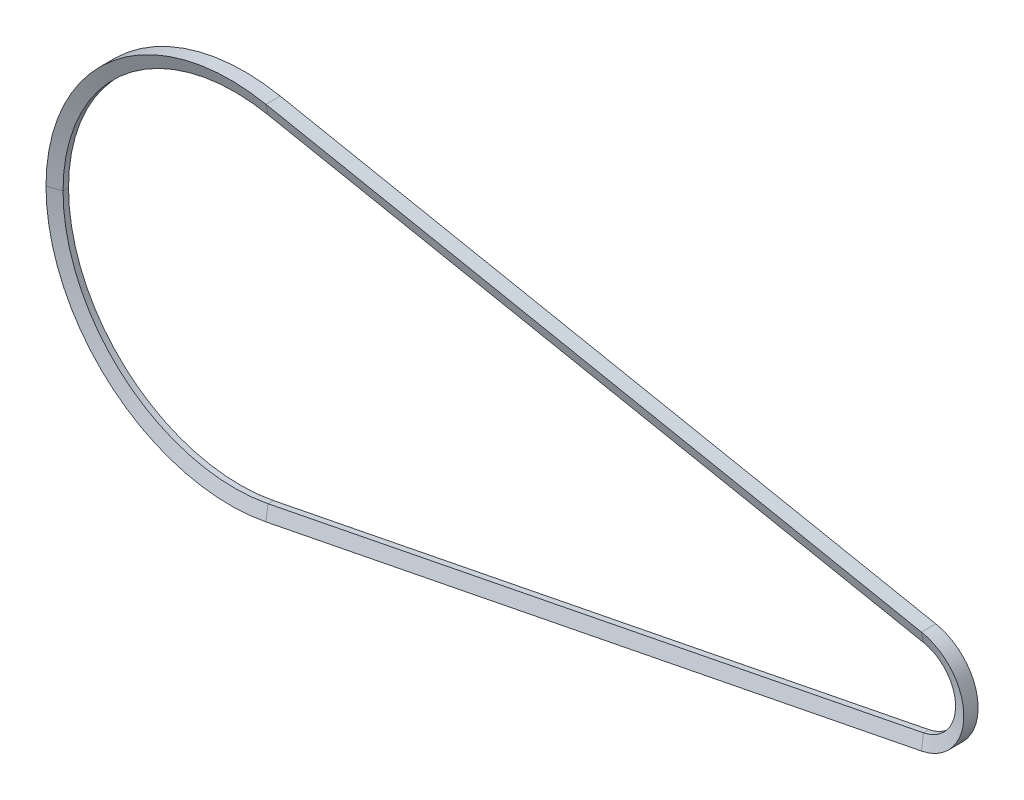
from build123d import *


with BuildPart() as part:
    # Sweep1: sweep along a path in Sketch1
    with BuildLine(Plane.XY) as sweep1_path:
        Line((30.251612903, 153.344481207), (627.025806452, 35.613593524))
        ThreePointArc((627.025806452, 35.613593524), (656.3, 0), (627.025806452, -35.613593524))
        Line((627.025806452, -35.613593524), (30.251612903, -153.344481207))
        ThreePointArc((30.251612903, -153.344481207), (-156.3, 0), (30.251612903, 153.344481207))
    # Sketch2 → Sweep1 (sweep)
    with BuildSketch(Plane(origin=(0, 0, 0), x_dir=(1, 0, 0), z_dir=(0, 1, 0))):
        Polygon((-156.3, 0), (-156.3, -5), (-167.8, -9), (-167.8, 4), align=None)
    sweep(path=sweep1_path.line)


solid = part.part
